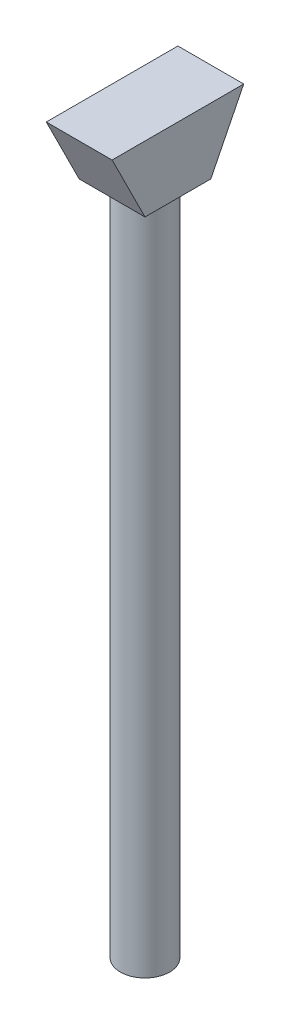
from build123d import *

# Parameters (mm, degrees)
SKETCH1_W               = 80
SKETCH1_H               = 40
BOSS_EXTRUDE1_DEPTH     = 20
CUT_EXTRUDE1_DEPTH      = 49.989794856
CUT_EXTRUDE1_DEPTH_BACK = 49.989794856
SKETCH3_R               = 15
BOSS_EXTRUDE2_DEPTH     = 410


with BuildPart() as part:
    # Sketch1 → Boss-Extrude1 (new, symmetric)
    with BuildSketch(Plane(origin=(0, 0, 0), x_dir=(0, 0, -1), z_dir=(1, 0, 0))):
        Rectangle(SKETCH1_W, SKETCH1_H)
    extrude(amount=BOSS_EXTRUDE1_DEPTH, both=True)

    # Sketch2 → Cut-Extrude1 (cut, two sides: drawn at the far end of the back side and taken through both)
    with BuildSketch(Plane(origin=(0, 0, 0), x_dir=(0, 0, -1), z_dir=(1, 0, 0)).offset(-CUT_EXTRUDE1_DEPTH_BACK)):
        Polygon((-40, 20), (-20, -20), (-40, -20), align=None)
        Polygon((40, 20), (40, -20), (20, -20), align=None)
    extrude(amount=CUT_EXTRUDE1_DEPTH + CUT_EXTRUDE1_DEPTH_BACK, mode=Mode.SUBTRACT)

    # Sketch3 → Boss-Extrude2 (add)
    with BuildSketch(Plane.XZ.offset(20)):
        with Locations(Location((0, 0, 0), (0, 0, 90))):
            Circle(SKETCH3_R)
    extrude(amount=BOSS_EXTRUDE2_DEPTH)


solid = part.part
